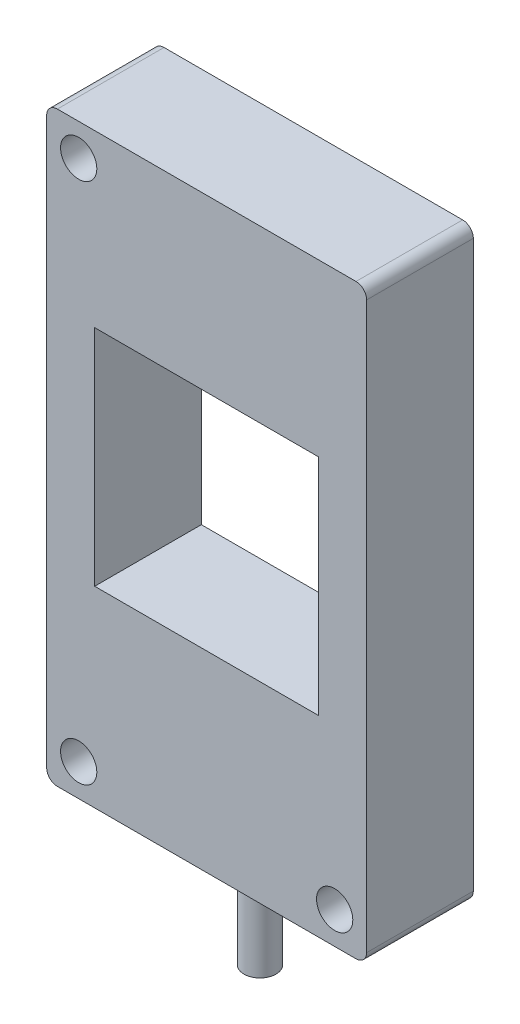
from build123d import *

# Parameters (mm, degrees)
SKETCH1_W                  = 30
SKETCH1_H                  = 55
BOSS_EXTRUDE1_DEPTH        = 5
SKETCH2_W                  = 21
SKETCH2_H                  = 21
CUT_EXTRUDE1_DEPTH         = 33.882366095
SKETCH3_R                  = 1.5
BOSS_EXTRUDE2_DEPTH        = 10
CHAMFER1_SIZE              = 1
FILLET1_R                  = 1
F_3_4_3_4_DIAMETER_HOLE1_D = 3.4


with BuildPart() as part:
    # Sketch1 → Boss-Extrude1 (new, symmetric)
    with BuildSketch(Plane.XY):
        Rectangle(SKETCH1_W, SKETCH1_H)
    extrude(amount=BOSS_EXTRUDE1_DEPTH, both=True)

    # Sketch2 → Cut-Extrude1 (cut, through all)
    with BuildSketch(Plane.XY.offset(5)):
        with Locations((0, 1)):
            Rectangle(SKETCH2_W, SKETCH2_H)
    extrude(amount=-CUT_EXTRUDE1_DEPTH, mode=Mode.SUBTRACT)

    # Sketch3 → Boss-Extrude2 (add)
    with BuildSketch(Plane.XZ.offset(27.5)):
        with Locations(Location((0, 0, 0), (0, 0, 90))):
            Circle(SKETCH3_R)
    extrude(amount=BOSS_EXTRUDE2_DEPTH)

    # Chamfer1
    chamfer1_edges = [part.edges().sort_by_distance(p)[0] for p in [
        (0, -27.5, -1.5),
    ]]
    chamfer(chamfer1_edges, length=CHAMFER1_SIZE)

    # Fillet1
    fillet1_edges = [part.edges().sort_by_distance(p)[0] for p in [
        (15, -27.5, 0),
        (-15, -27.5, 0),
        (-15, 27.5, 0),
        (15, 27.5, 0),
    ]]
    fillet(fillet1_edges, radius=FILLET1_R)

    # Ø3.4 (3.4) Diameter Hole1 (through all)
    with Locations(Plane.XY.offset(5)):
        with Locations((-12, 24.5), (-12, -24.5), (12, -24.5)):
            Hole(F_3_4_3_4_DIAMETER_HOLE1_D / 2)


solid = part.part
